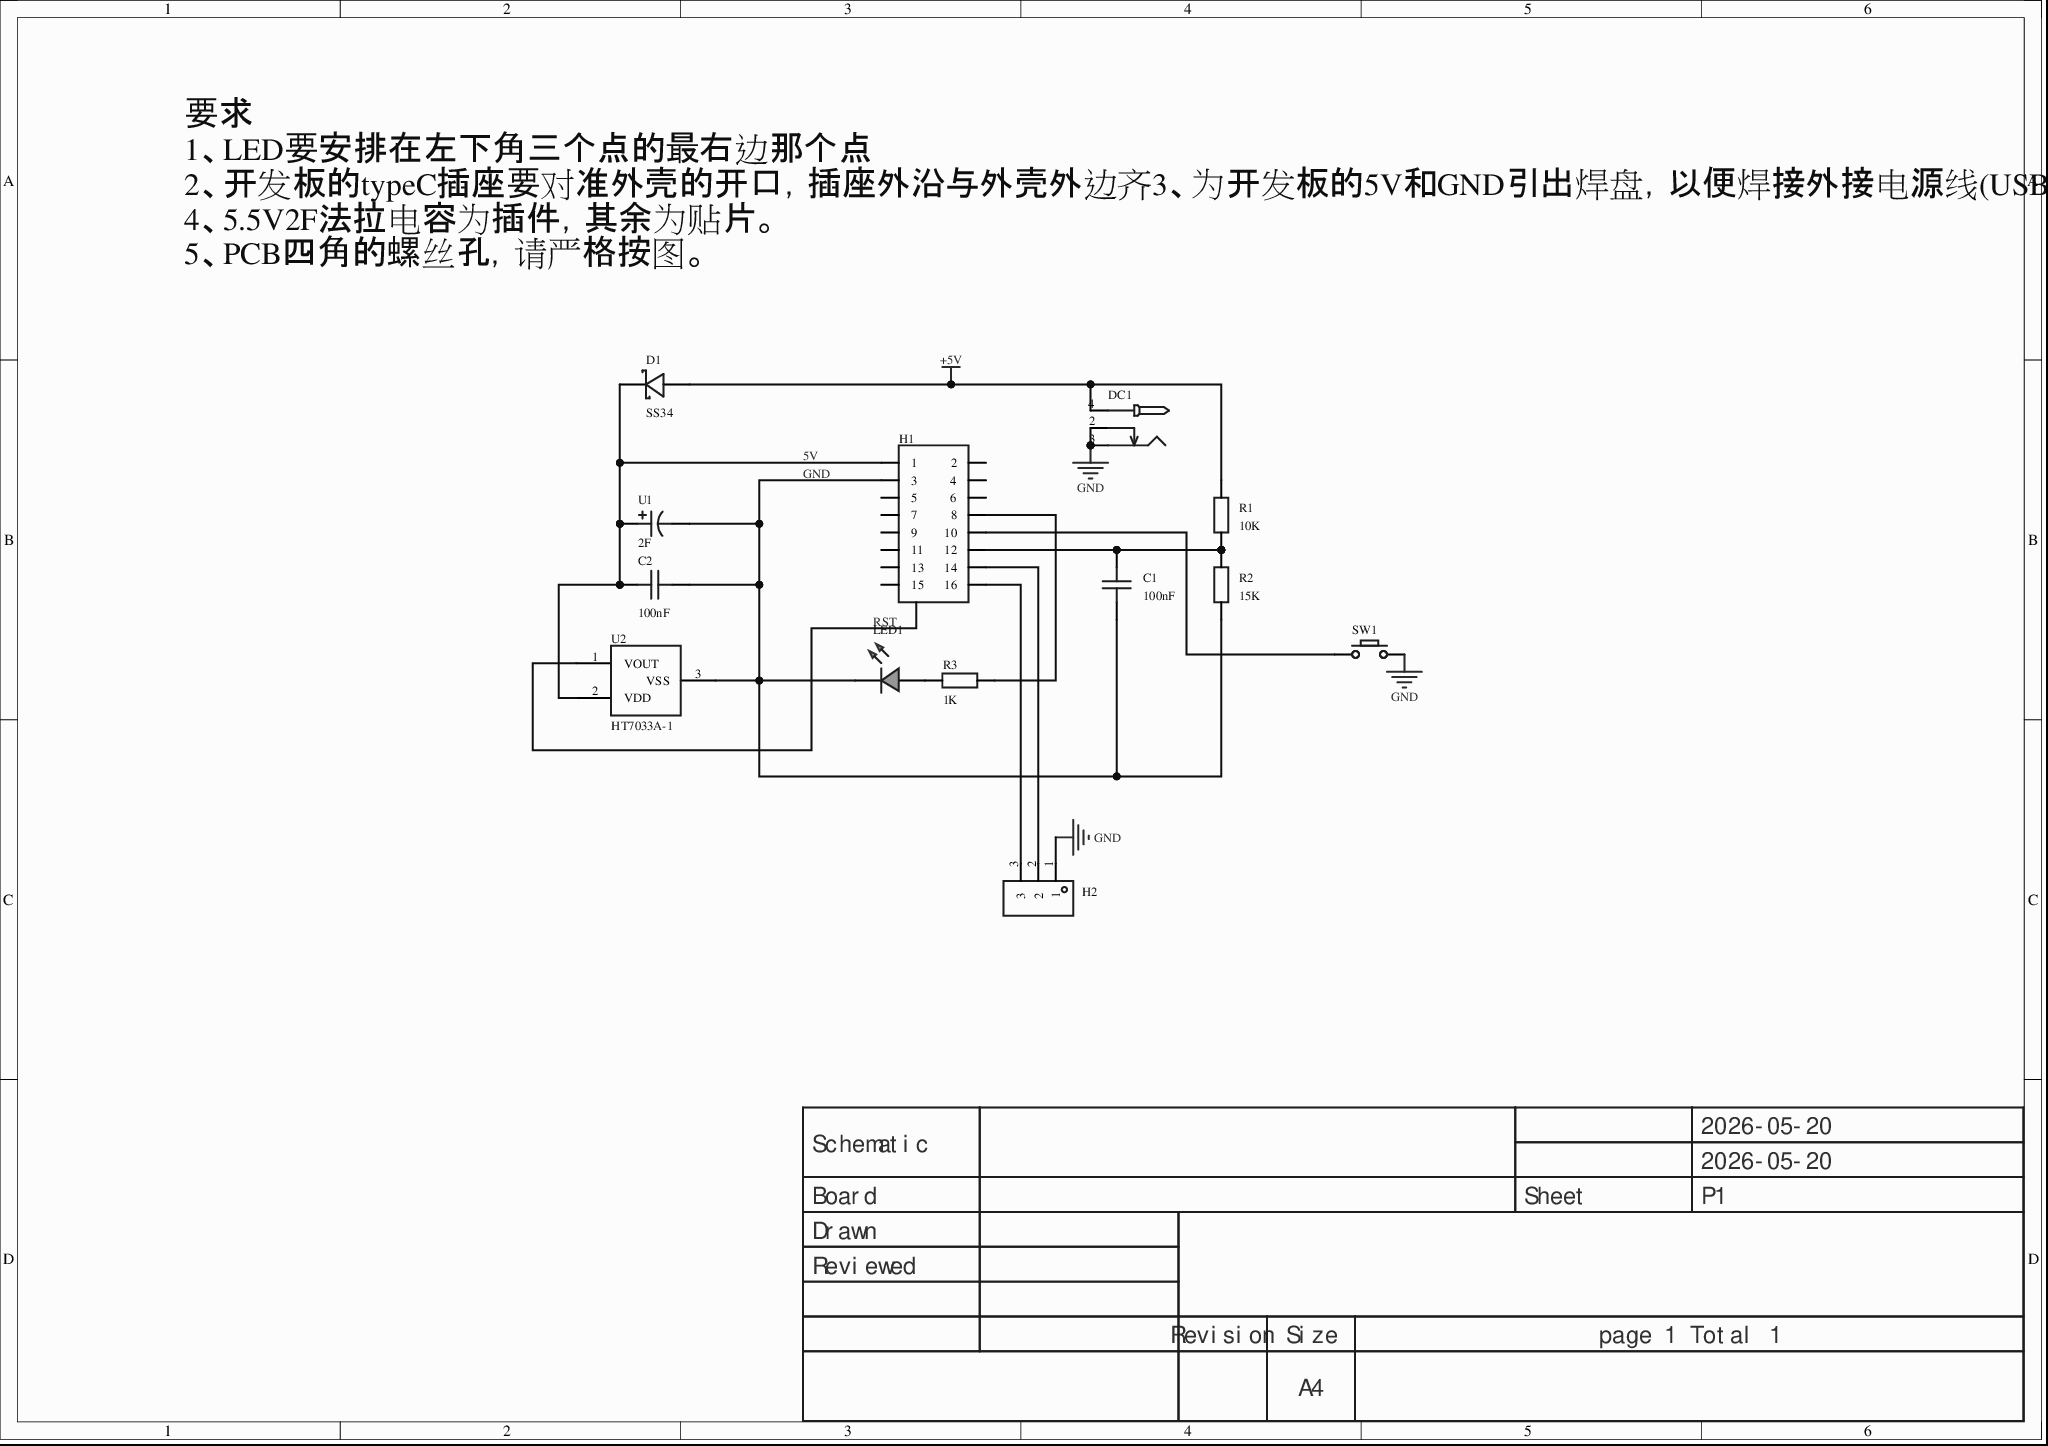
[diagram p0: MISC52083-3.schdoc]
# Altium project MISC52083-2.PrjPcb
1 sheet, 13 parts. Net scope: global (net labels, ports and power ports of the same name join across sheets).
Board file: MISC52083.pcbdoc

## Sheet MISC52083-3.schdoc
size 297 x 209 mm; Version: V1.0; @Project Name: MISC52083; @Update Date: 2026-05-20; @Create Date: 2026-05-20; @Board Name: MISC52083; @Create Time: 10:48:44; @Page Count: 1; @Page No: 1; @Schematic Name: MISC52083; @Update Time: 10:48:44; Size: A4

### Parts
C1  100nF  [C0603]
C2  100nF  [C0603]
D1  SS34  [SMA_L4.3-W2.6-LS5.2-RD]
DC1  (no value)  [DC-2.0]
H1  (no value)  [HDR-TH_16P-P2.54-V-F-R2-C8-S2.54-1]
H2  (no value)  [HDR-TH_3P-P2.54-V-M]
LED1  (no value)  [LED_0603]
R1  10K  [R0603]
R2  15K  [R0603]
R3  1K  [R0603]
SW1  (no value)  [Key_TH_3.5x6x4.3]
U1  2F  [CAP-TH_BD8.0-P3.50-D0.6-FD_GDC02R7R205LD0816]
U2  HT7033A-1  [SOT-89-3_L4.5-W2.5-P1.50-LS4.2-BR]

### Nets
+5V: D1.2(A) DC1.4 R1.2
GND: C1.1 C2.1 DC1.2 DC1.3 H1.3 H2.1 LED1.1(C) R2.1 SW1.B U1.2 U2.3(VSS)
5V: C2.2 D1.1(K) H1.1 U1.1 U2.2(VDD)
RST: U2.1(VOUT)
NetC1_2: C1.2 H1.12 R1.1 R2.2
NetH1_8: H1.8 R3.1
NetH1_10: H1.10 SW1.A
NetH1_14: H1.14 H2.2
NetH1_16: H1.16 H2.3
NetLED1_2: LED1.2(A) R3.2

Not connected (* = marked no-connect by the designer): H1 2 4 5 6 7 9 11 13 15

### Notes on the sheet
- 要求
  1、LED要安排在左下角三个点的最右边那个点
  2、开发板的typeC插座要对准外壳的开口，插座外沿与外壳外边齐3、为开发板的5V和GND引出焊盘，以便焊接外接电源线(USB二芯线)
  4、5.5V2F法拉电容为插件，其余为贴片。
  5、PCB四角的螺丝孔，请严格按图。
- 2026-05-20
- Schematic
- Board
- Sheet
- P1
- Drawn
- Reviewed
- Revision
- Size
- A4
- page 1 Total 1

### Library data of the parts
C1 C2 = CAP_0603: Symbol: Capacitance; ConvertToPcb: yes; ModelId: ac125912035d415993ca9572d50418b10819f05c4eef4c71ace90d822a990e87; ModelName: C0603_L1.6-W0.8-H0.8; ModelTransform: 62.992,31.496,0,0,0,0,0,0,0; Device: CAP_0603; AddInBom: yes; Supplier Footprint: 0603; FootprintName: C0603; Value: 100nF
D1 = SS34_C8678: Diode configuration:Single;Forward voltage(Vf):550mV@3A;Reverse voltage(Vr):40V;Rectified current:3A;; Manufacturer: MDD(辰达半导体); AddInBom: yes; ModelId: e3551acb3c5a4975a5e9d36087fe1fa20819f05c4eef4c71ace90d822a990e87; ModelTransform: 185.039,102.362,0,0,0,0,0,0,0; Diode Configuration: Single; Voltage - DC Reverse(Vr): 40V; Current - Rectified: 3A; Reverse Leakage Current (Ir): 500uA@40V; Operating Junction Temperature Range: -55℃~+125℃; Symbol: SS34_C8678; Device: SS34_C8678; LCSC Part Name: 电压:40V 电流:3A; SupplierPart: C8678; ManufacturerPart: SS34; Supplier Footprint: SMA(DO-214AC); JLCPCB Part Class: Basic Part; Datasheet: https://item.szlcsc.com/datasheet/SS34/9178.html; Supplier: LCSC; ConvertToPcb: yes; FootprintName: SMA_L4.3-W2.6-LS5.2-RD; ModelName: SMA_L4.3-W2.6-LS5.2-RD; Voltage - Forward(Vf@If): 550mV@3A
DC1 = DC-005_2.0: Symbol: DC power connector; ConvertToPcb: yes; ModelId: f5f20b8a2308479b936ba3c2698865bb0819f05c4eef4c71ace90d822a990e87; ModelName: DC-IN-TH_DC-5520-1; ModelTransform: 372.05,551.18,582.68,90,0,0,137.8,0,-149.61; Device: DC-005_2.0; AddInBom: yes; Supplier Footprint: 插件; FootprintName: DC-2.0
H1 = HDR-F_2.54_2x8: Symbol: HDR-F-2.54_2x8; ConvertToPcb: yes; ModelId: f6b5f7d40ec74b809fbaeebc5002f6e00819f05c4eef4c71ace90d822a990e87; ModelName: HDR2.54-F-LI-2X8P; ModelTransform: 799.99844,200,0,0,0,0,0,0,-118.11; Device: HDR-F_2.54_2x8; AddInBom: yes; SupplierPart: C30734; Supplier Footprint: 插件; FootprintName: HDR-TH_16P-P2.54-V-F-R2-C8-S2.54-1
H2 = HDR-M_2.54_1x3P: AddInBom: yes; ModelId: bb473b6d38ff42a99216a4fcdbdcc4cb0819f05c4eef4c71ace90d822a990e87; ModelName: HDR-TH_3P-P2.54-M-LI-1X3P; ModelTransform: 300.03877,100,0,0,0,0,0,0,-118.11; Symbol: HDR-M_2.54_1x3P; Device: HDR-M_2.54_1x3P; ConvertToPcb: yes; FootprintName: HDR-TH_3P-P2.54-V-M; SupplierPart: C2937625; Supplier Footprint: 插件
LED1 = LED_0603-G: Symbol: LED_G_OLD; Convert to PCB: yes; 3D Model: 8b5fcaf0229049f8a37a9c352bb0ca0a0819f05c4eef4c71ace90d822a990e87; 3D Model Transform: 63.1,31.6,23.7,0,0,0,0,0,0; ModelName: LED-0603_G; Device: LED_0603-G; Add into BOM: yes; Supplier Footprint: 0603; FootprintName: LED_0603
R1-R3 = Res_0603: Symbol: Resistor; ConvertToPcb: yes; ModelId: fc143cca1e79419f9cd78b61e9279f080819f05c4eef4c71ace90d822a990e87; ModelTransform: 31.8897,63.7794,0,90,0,0,0,0,0; Device: Res_0603; AddInBom: yes; Supplier Footprint: 0603; FootprintName: R0603; ModelName: R0603
  R1: Value: 10K
  R2: Value: 15K
  R3: Value: 1K
SW1 = Key_TH_3.5x6x4.3: ConvertToPcb: yes; ModelId: c3523f9014d949d7ba5445190a3178990819f05c4eef4c71ace90d822a990e87; ModelName: SW-TH_L6.0-W3.5-H5.0-P6.5; ModelTransform: 308.49,137.8,335.08,0,0,0,0,0,-129.92; Symbol: Key_TH_3.5x6x4.3; Device: Key_TH_3.5x6x4.3; AddInBom: yes; Supplier Footprint: 插件; FootprintName: Key_TH_3.5x6x4.3
U1 = GDC02R7R205LD0816: Capacitance:2F;Tolerance:-20%~+50%;Rated voltage:2.7V;Leakage current:10uA@72hrs;ESR:100mΩ@1kHz;; Manufacturer: GODETEK(皋德科技); AddInBom: yes; Voltage Rating: 2.7V; Lifetime: 1000hrs@70℃; Cycle Life Expectancy: 50 ten-thousand cycles; Symbol: GDC02R7R205LD0816; Device: GDC02R7R205LD0816; LCSC Part Name: 2F -20%~+50% 2.7V; SupplierPart: C24833981; ManufacturerPart: GDC02R7R205LD0816; Supplier Footprint: 插件,D8xL16mm; Datasheet: https://item.szlcsc.com/datasheet/GDC02R7R205LD0816/26563160.html; Supplier: LCSC; ConvertToPcb: yes; FootprintName: CAP-TH_BD8.0-P3.50-D0.6-FD_GDC02R7R205LD0816; Value: 2F; Tolerance: -20%~+50%; Current - Leakage: 10uA@72hrs; Equivalent Series Resistance(ESR): 100mΩ@1kHz; Operating Temperature: -40℃~+70℃; Diameter: 8mm; Height - Seated(Max): 16mm
U2 = HT7033A-1_C73715: Operating voltage:1.5V~30V;Reset active level:Active low;Monitored voltage count:1;Reset timeout:200us;; Manufacturer: HOLTEK(合泰/盛群); AddInBom: yes; ModelId: 6db690b7897d4d18a30d90c1b89525ee0819f05c4eef4c71ace90d822a990e87; ModelName: SOT-89-3_L4.3-W2.5-H1.6-LS4.1-P1.50; ModelTransform: 161.417,169.291,0,180,0,0,-11.808,0,0; ChipType: Voltage detector; Output Type: Open drain; Threshold Voltage: 3.3V; Number of Voltages Monitored: 1; Reset Timeout: 200us; Quiescent Current: 3uA; Symbol: HT7033A-1; Device: HT7033A-1_C73715; LCSC Part Name: HT7033A-1; SupplierPart: C73715; ManufacturerPart: HT7033A-1; Supplier Footprint: SOT-89-3; JLCPCB Part Class: Extended Part; Datasheet: https://www.holtek.com.cn/webapi/116706/simHT70xxA-1v260.pdf; Supplier: LCSC; ConvertToPcb: yes; FootprintName: SOT-89-3_L4.5-W2.5-P1.50-LS4.2-BR; Voltage - Supply: 1.5V~30V; Reset Active Level: Active low; Operating Temperature: -40℃~+85℃@(TA)